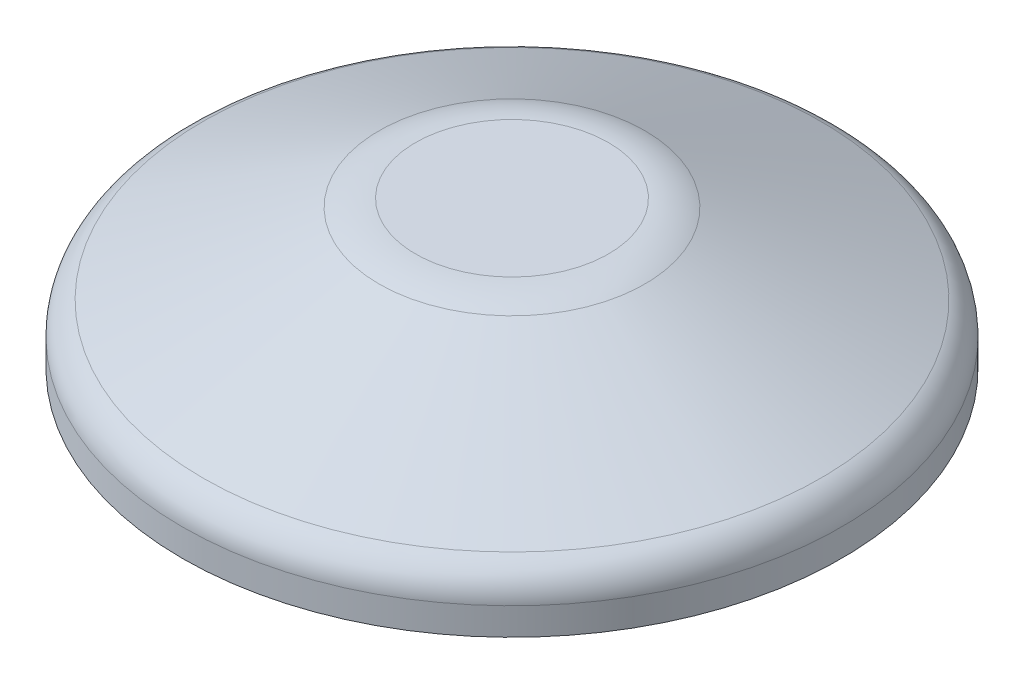
SolidWorks part; units mm, degrees
ref_plane "Front Plane" through (0, 0, 0) normal (0, 0, 1) x (1, 0, 0)
ref_plane "Top Plane" through (0, 0, 0) normal (0, 1, 0) x (1, 0, 0)
ref_plane "Right Plane" through (0, 0, 0) normal (1, 0, 0) x (0, 0, -1)
sketch "Sketch1" plane through (0, 0, 0) normal (0, 0, 1) x (1, 0, 0)
  line L0 (0, 0) -> (0, 67.3496) construction
  line L1 (-150, 1.448) -> (-150, 24.1749)
  line L2 (-138, 1.448) -> (-138, 16.448) construction
  line L3 (-138, 16.448) -> (-50, 56.448) construction
  line L4 (-50, 56.448) -> (0, 56.448)
  line L5 (-150, 24.1749) -> (-52.5993, 68.448)
  line L6 (-52.5993, 68.448) -> (0, 68.448)
  line L7 (-150, 1.448) -> (-138, 1.448)
  line L8 (-138, 1.448) -> (-132, 1.448) construction
  line L9 (-132, 1.448) -> (-132, 19.1753)
  line L10 (-132, 19.1753) -> (-50, 56.448)
  line L11 (-138, 1.448) -> (-138, -4.552)
  line L12 (-138, -4.552) -> (-132, -4.552)
  line L13 (-132, -4.552) -> (-132, 1.448)
  line L14 (0, 68.448) -> (0, 56.448)
  dimension "D1" = 55
  dimension "D2" = 15
  dimension "D3" = 50
  dimension "D4" = 138
  dimension "D6" = 6
  dimension "D7" = 6
  dimension "D5" = 12
revolve "Revolve1" add sketch "Sketch1" angle 360 about L0
fillet "Fillet1" radius 40 1 edges at (0, 68.448, -52.5993)
fillet "Fillet2" radius 38 1 edges at (0, 56.448, -50)
fillet "Fillet3" radius 16 1 edges at (0, 24.1749, -150)
fillet "Fillet4" radius 4 1 edges at (0, 19.1753, -132)
